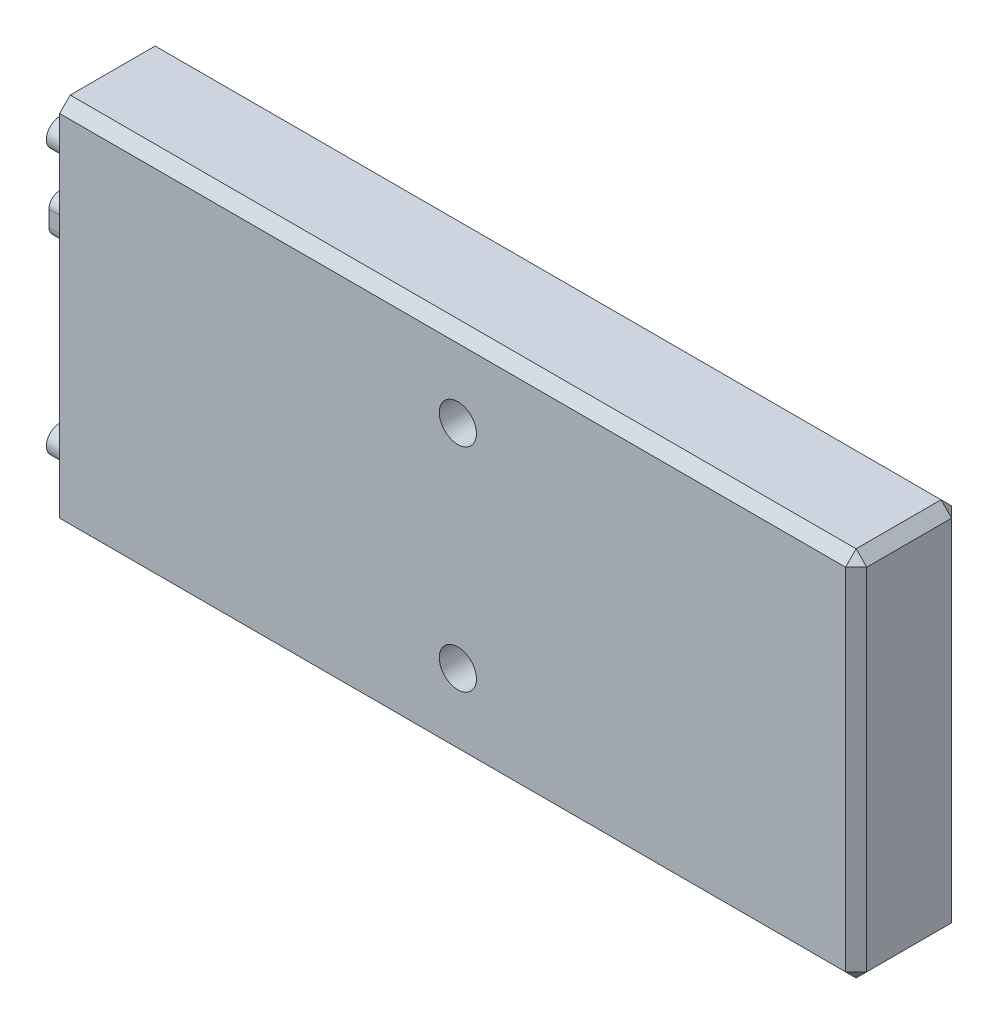
from build123d import *

# Parameters (mm, degrees)
SKETCH2_W           = 150
SKETCH2_H           = 70
BOSS_EXTRUDE1_DEPTH = 10
SKETCH3_R           = 2.5
SKETCH3_R_2         = 1
SKETCH3_W           = 3
SKETCH3_H           = 6
BOSS_EXTRUDE2_DEPTH = 5
CHAMFER1_SIZE       = 2
SKETCH4_R           = 3.5
CUT_EXTRUDE1_DEPTH  = 90.582364336


with BuildPart() as part:
    # Sketch2 → Boss-Extrude1 (new, symmetric)
    with BuildSketch(Plane.XY):
        Rectangle(SKETCH2_W, SKETCH2_H)
    extrude(amount=BOSS_EXTRUDE1_DEPTH, both=True)

    # Sketch3 → Boss-Extrude2 (add)
    # profile 1 of 6: a face of its own
    with BuildSketch(Plane.ZY.offset(75)):
        with Locations(Location((-5, -25, 0), (0, 0, 90))):
            Circle(SKETCH3_R)
        with Locations(Location((-5, -25, 0), (0, 0, 270))):
            Circle(SKETCH3_R_2, mode=Mode.SUBTRACT)
    # profile 2 of 6: a face of its own
    with BuildSketch(Plane.ZY.offset(75)):
        with Locations(Location((5, -25, 0), (0, 0, 90))):
            Circle(SKETCH3_R)
        with Locations(Location((5, -25, 0), (0, 0, 270))):
            Circle(SKETCH3_R_2, mode=Mode.SUBTRACT)
    # profile 3 of 6: a face of its own
    with BuildSketch(Plane.ZY.offset(75)):
        with Locations(Location((5, 25, 0), (0, 0, 90))):
            Circle(SKETCH3_R)
        with Locations(Location((5, 25, 0), (0, 0, 90))):
            Circle(SKETCH3_R_2, mode=Mode.SUBTRACT)
    # profile 4 of 6: a face of its own
    with BuildSketch(Plane.ZY.offset(75)):
        with Locations(Location((-5, 25, 0), (0, 0, 90))):
            Circle(SKETCH3_R)
        with Locations(Location((-5, 25, 0), (0, 0, 90))):
            Circle(SKETCH3_R_2, mode=Mode.SUBTRACT)
    # profile 5 of 6: a face of its own
    with BuildSketch(Plane.ZY.offset(75)):
        with BuildLine():
            Line((7, 13.4135929), (7, 10.4135929))
            ThreePointArc((7, 10.4135929), (5, 8.4135929), (3, 10.4135929))
            Line((3, 10.4135929), (3, 13.4135929))
            ThreePointArc((3, 13.4135929), (5, 15.4135929), (7, 13.4135929))
        make_face()
    # profile 6 of 6: a face of its own
    with BuildSketch(Plane.ZY.offset(75)):
        with Locations((-5, 12)):
            Rectangle(SKETCH3_W, SKETCH3_H)
    extrude(amount=BOSS_EXTRUDE2_DEPTH)

    # Chamfer1
    chamfer1_edges = [part.edges().sort_by_distance(p)[0] for p in [
        (0, -35, 10),
        (75, 0, 10),
        (0, -35, -10),
        (0, 35, -10),
        (75, 0, -10),
        (75, -35, 0),
        (-75, -35, 0),
        (75, 35, 0),
        (0, 35, 10),
    ]]
    chamfer(chamfer1_edges, length=CHAMFER1_SIZE)

    # Sketch4 → Cut-Extrude1 (cut, through all)
    with BuildSketch(Plane.XY.offset(10)):
        with Locations((0, 20)):
            Circle(SKETCH4_R)
        with Locations((0, -20)):
            Circle(SKETCH4_R)
    extrude(amount=-CUT_EXTRUDE1_DEPTH, mode=Mode.SUBTRACT)


solid = part.part
